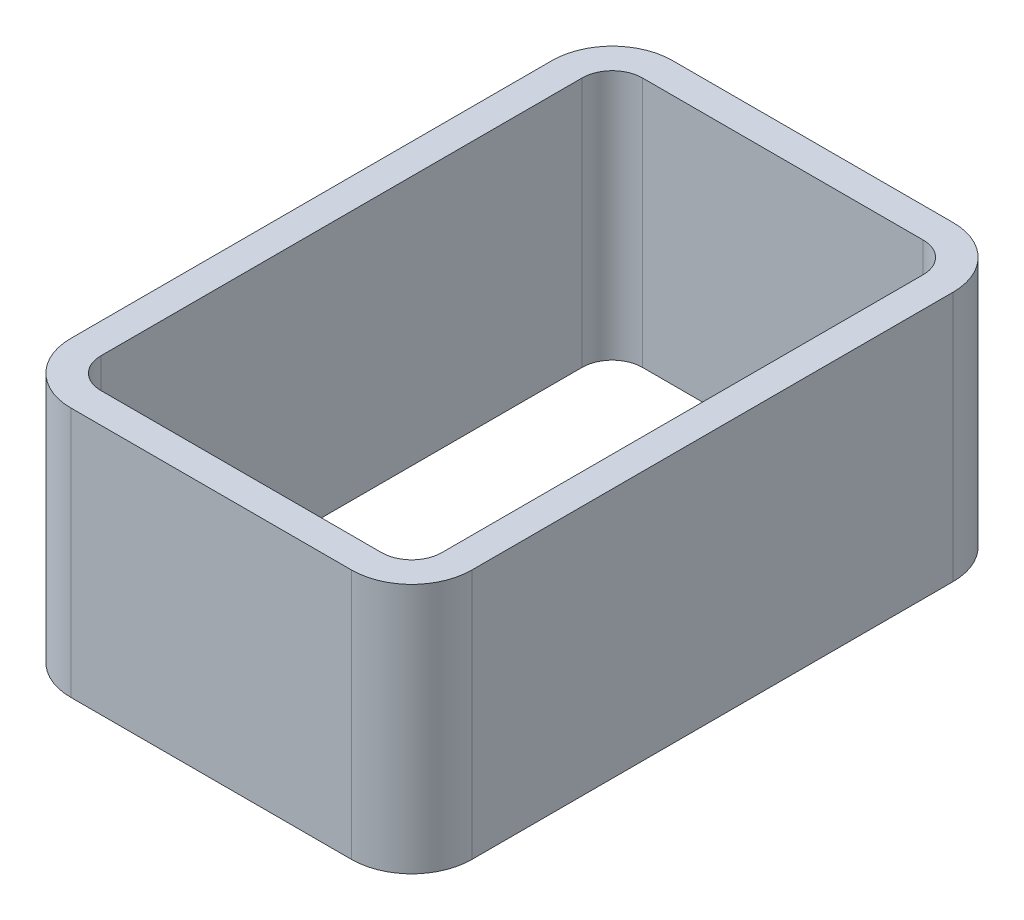
SolidWorks part; units mm, degrees
material "Q235B"
ref_plane "Front Plane" through (0, 0, 0) normal (0, 0, 1) x (1, 0, 0)
ref_plane "Top Plane" through (0, 0, 0) normal (0, 1, 0) x (1, 0, 0)
ref_plane "Right Plane" through (0, 0, 0) normal (1, 0, 0) x (0, 0, -1)
sketch "Sketch1" plane through (0, 0, 0) normal (0, 0, 1) x (1, 0, 0)
  line L0 (0, 0) -> (0, 25)
  dimension "D1" = 25
other "GB/T 6728-2002 Rectangular Hollow Section 60X40X3(1)"
ref_plane "Plane1" through (0, 0, 0) normal (0, 1, 0) x (-1, 0, 0)
sketch "Sketch13" plane through (0, 0, 0) normal (0, 1, 0) x (-1, 0, 0)
  line L0 (-14, -27) -> (14, -27)
  line L1 (-17, -24) -> (-17, 24)
  line L2 (14, 27) -> (-14, 27)
  line L3 (17, 24) -> (17, -24)
  line L4 (-14, -30) -> (14, -30)
  line L5 (-20, -24) -> (-20, 24)
  line L6 (14, 30) -> (-14, 30)
  line L7 (20, 24) -> (20, -24)
  arc A0 (20, 24) -> (14, 30) centre (14, 24) ccw
  arc A1 (14, -30) -> (20, -24) centre (14, -24) ccw
  arc A2 (-20, -24) -> (-14, -30) centre (-14, -24) ccw
  arc A3 (-14, 30) -> (-20, 24) centre (-14, 24) ccw
  arc A4 (-14, 27) -> (-17, 24) centre (-14, 24) ccw
  arc A5 (17, 24) -> (14, 27) centre (14, 24) ccw
  arc A6 (14, -27) -> (17, -24) centre (14, -24) ccw
  arc A7 (-17, -24) -> (-14, -27) centre (-14, -24) ccw
  point P0 (0, 30)
  point P1 (20, 0)
  point P2 (0, -30)
  point P3 (-20, 0)
  point P4 (-20, 30)
  point P5 (20, 30)
  point P6 (20, -30)
  point P7 (-20, -30)
  point P8 (0, 0)
  point P33 (0, 0)
  dimension "D1" = 6
  dimension "Thickness" = 3
  dimension "V_leg" = 60
  dimension "H_leg" = 40
